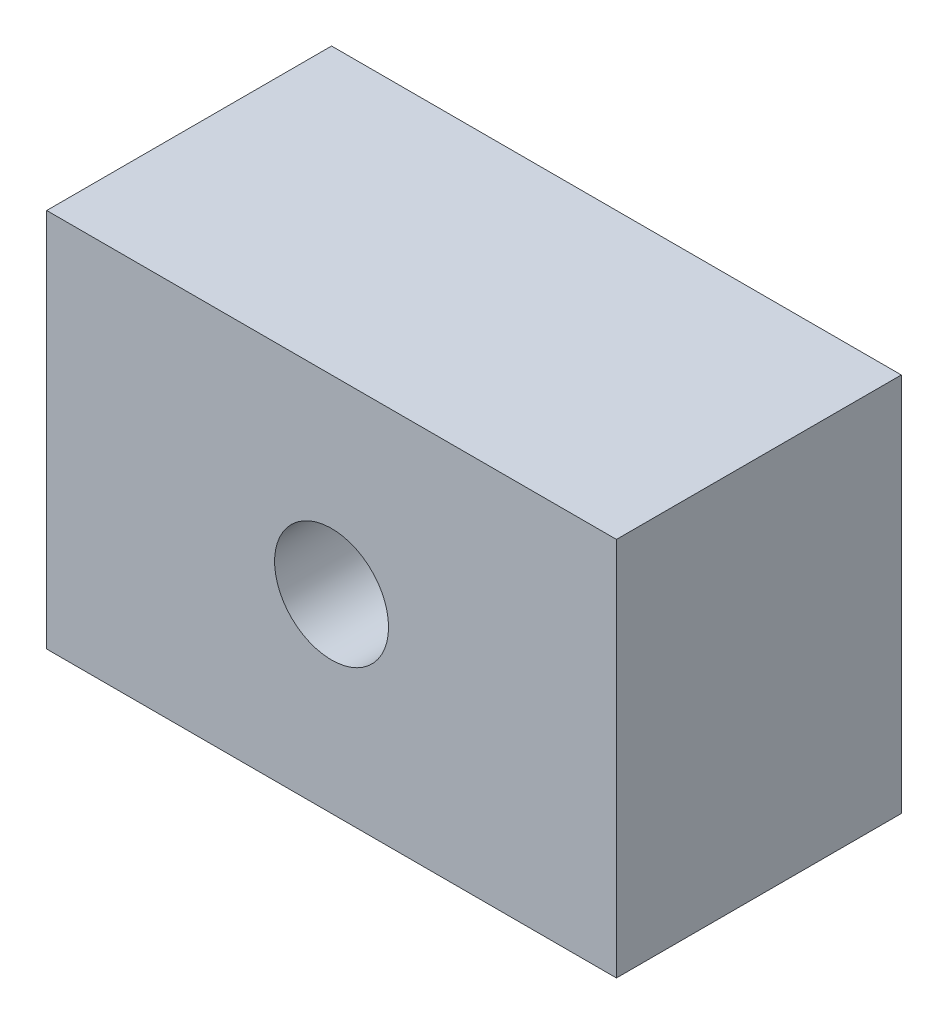
from build123d import *

# Parameters (mm, degrees)
SKETCH1_W               = 30
SKETCH1_H               = 20
BOSS_EXTRUDE1_DEPTH     = 15
CUT_EXTRUDE1_DEPTH      = 24.452078799
CUT_EXTRUDE1_DEPTH_BACK = 24.452078799
SKETCH2_R               = 3


with BuildPart() as part:
    # Sketch1 → Boss-Extrude1 (new body)
    with BuildSketch(Plane.XY):
        Rectangle(SKETCH1_W, SKETCH1_H)
    extrude(amount=BOSS_EXTRUDE1_DEPTH)

    # Sketch2 → Cut-Extrude1 (cut, two sides: drawn at the far end of the back side and taken through both)
    with BuildSketch(Plane.XY.offset(15).offset(-CUT_EXTRUDE1_DEPTH_BACK)):
        Circle(SKETCH2_R)
    extrude(amount=CUT_EXTRUDE1_DEPTH + CUT_EXTRUDE1_DEPTH_BACK, mode=Mode.SUBTRACT)


solid = part.part
